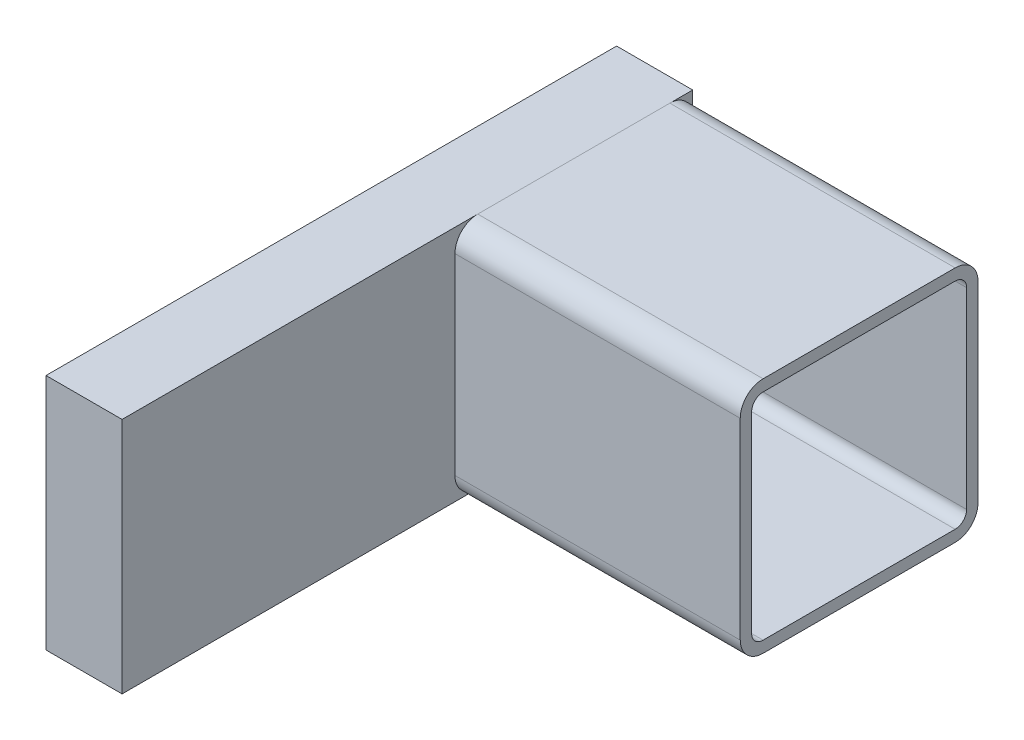
SolidWorks part; units mm, degrees
ref_plane "Front Plane" through (0, 0, 0) normal (0, 0, 1) x (1, 0, 0)
ref_plane "Top Plane" through (0, 0, 0) normal (0, 1, 0) x (1, 0, 0)
ref_plane "Right Plane" through (0, 0, 0) normal (1, 0, 0) x (0, 0, -1)
sketch "草图1" plane through (0, 0, 0) normal (0, 1, 0) x (1, 0, 0)
  line L0 (-15, 0) -> (15, 0)
  line L2 (0, 0) -> (0, 66.6058) construction
  point P4 (0, 0)
  dimension "D1" = 30
other "Gb／6728-1986 square hollow section 025 X 25 X 1.2(1)"
ref_plane "Plane1" through (-15, 0, 0) normal (1, 0, 0) x (0, 0, -1)
sketch "Sketch1" plane through (-15, 0, 0) normal (1, 0, 0) x (0, 0, -1)
  line L0 (-10.1, -11.3) -> (10.1, -11.3)
  line L1 (-11.3, -10.1) -> (-11.3, 10.1)
  line L2 (10.1, 11.3) -> (-10.1, 11.3)
  line L3 (11.3, 10.1) -> (11.3, -10.1)
  line L4 (-10.1, -12.5) -> (10.1, -12.5)
  line L5 (-12.5, -10.1) -> (-12.5, 10.1)
  line L6 (10.1, 12.5) -> (-10.1, 12.5)
  line L7 (12.5, 10.1) -> (12.5, -10.1)
  arc A0 (12.5, 10.1) -> (10.1, 12.5) centre (10.1, 10.1) ccw
  arc A1 (10.1, -12.5) -> (12.5, -10.1) centre (10.1, -10.1) ccw
  arc A2 (-12.5, -10.1) -> (-10.1, -12.5) centre (-10.1, -10.1) ccw
  arc A3 (-10.1, 12.5) -> (-12.5, 10.1) centre (-10.1, 10.1) ccw
  arc A4 (-10.1, 11.3) -> (-11.3, 10.1) centre (-10.1, 10.1) ccw
  arc A5 (11.3, 10.1) -> (10.1, 11.3) centre (10.1, 10.1) ccw
  arc A6 (10.1, -11.3) -> (11.3, -10.1) centre (10.1, -10.1) ccw
  arc A7 (-11.3, -10.1) -> (-10.1, -11.3) centre (-10.1, -10.1) ccw
  point P0 (-12.5, 0)
  point P1 (12.5, 0)
  point P2 (0, 12.5)
  point P3 (0, -12.5)
  point P4 (0, 0)
  point P5 (-12.5, -12.5)
  point P6 (12.5, -12.5)
  point P7 (12.5, 12.5)
  point P8 (-12.5, 12.5)
  point P33 (0, 0)
  dimension "D1" = 2.4
  dimension "Thickness" = 1.2
  dimension "V_leg" = 25
sketch "Sketch3" plane through (-15, 0, 0) normal (-1, 0, 0) x (0, 0, 1)
  line L0 (-12.5, -10.1) -> (-12.5, 10.1) construction
  line L1 (-12.5, 12.5) -> (47.5, 12.5)
  line L2 (-12.5, 12.5) -> (-12.5, -12.5)
  line L3 (-12.5, -12.5) -> (47.5, -12.5)
  line L4 (47.5, 12.5) -> (47.5, -12.5)
  line L5 (-10.1, 12.5) -> (10.1, 12.5) construction
  line L6 (10.1, -12.5) -> (-10.1, -12.5) construction
  dimension "D1" = 60
extrude "Boss-Extrude1" add sketch "Sketch3" along normal blind 8 separate body
